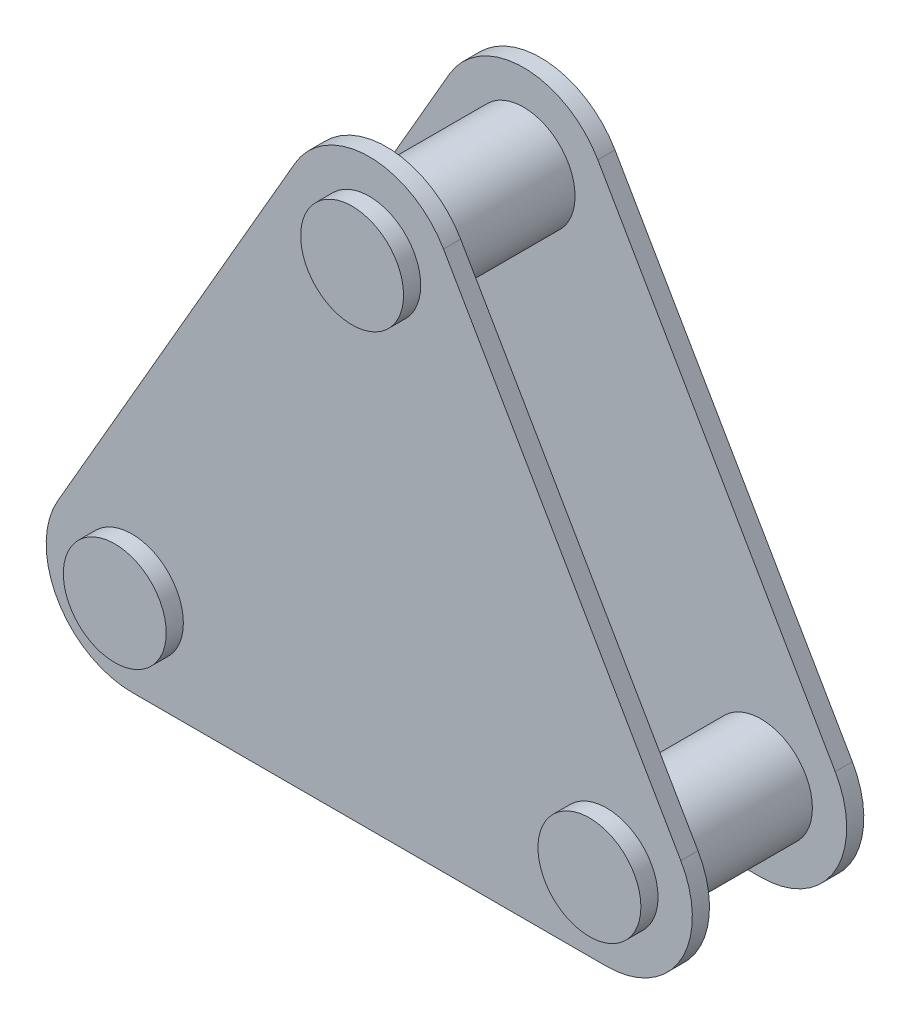
SolidWorks part; units mm, degrees
ref_plane "Front Plane" through (0, 0, 0) normal (0, 0, 1) x (1, 0, 0)
ref_plane "Top Plane" through (0, 0, 0) normal (0, 1, 0) x (1, 0, 0)
ref_plane "Right Plane" through (0, 0, 0) normal (1, 0, 0) x (0, 0, -1)
sketch "Sketch1" plane through (0, 0, 0) normal (0, 0, 1) x (1, 0, 0)
  line L1 (18.1699, -5.4904) -> (4.3301, 18.4808)
  line L2 (-4.3301, 18.4808) -> (-18.1699, -5.4904)
  line L3 (-13.8397, -12.9904) -> (13.8397, -12.9904)
  circle A0 centre (0, 15.9808) radius 3
  arc A1 (13.8397, -12.9904) -> (18.1699, -5.4904) centre (13.8397, -7.9904) ccw
  arc A2 (-13.8397, -12.9904) -> (-18.1699, -5.4904) centre (-13.8397, -7.9904) cw
  arc A3 (4.3301, 18.4808) -> (-4.3301, 18.4808) centre (0, 15.9808) ccw
  circle A4 centre (13.8397, -7.9904) radius 3
  circle A5 centre (-13.8397, -7.9904) radius 3
  point P8 (22.5, -12.9904)
  point P11 (-22.5, -12.9904)
  point P19 (0, 0)
  dimension "D2" = 5
  dimension "D3" = 6
  dimension "D1" = 45
  dimension "D4" = 3
extrude "Boss-Extrude1" add sketch "Sketch1" along normal blind 1
sketch "Sketch2" plane through (0, 0, 1) normal (0, 0, 1) x (1, 0, 0)
  circle A0 centre (13.8397, -7.9904) radius 3 construction
  circle A1 centre (-13.8397, -7.9904) radius 3 construction
  circle A2 centre (0, 15.9808) radius 3 construction
  circle A3 centre (13.8397, -7.9904) radius 3
  circle A4 centre (-13.8397, -7.9904) radius 3
  circle A5 centre (0, 15.9808) radius 3
extrude "Boss-Extrude2" add sketch "Sketch2" against normal blind 11
ref_plane "Plane3" through (0, 0, -4.5) normal (0, 0, -1) x (-1, 0, 0)
ref_plane "Plane4" through (0, 0, -4) normal (0, 0, -1) x (-1, 0, 0)
mirror "Mirror3" about plane through (0, 0, -4) normal (0, 0, -1) of "Boss-Extrude1"
sketch "Sketch3" plane through (0, 0, 1) normal (0, 0, 1) x (1, 0, 0)
  circle A0 centre (0, 15.9808) radius 3
  circle A1 centre (13.8397, -7.9904) radius 3
  circle A2 centre (-13.8397, -7.9904) radius 3
  point P9 (0, 0)
  dimension "D1" = 6
  dimension "D2" = 3
extrude "Boss-Extrude3" add sketch "Sketch3" along normal blind 1
